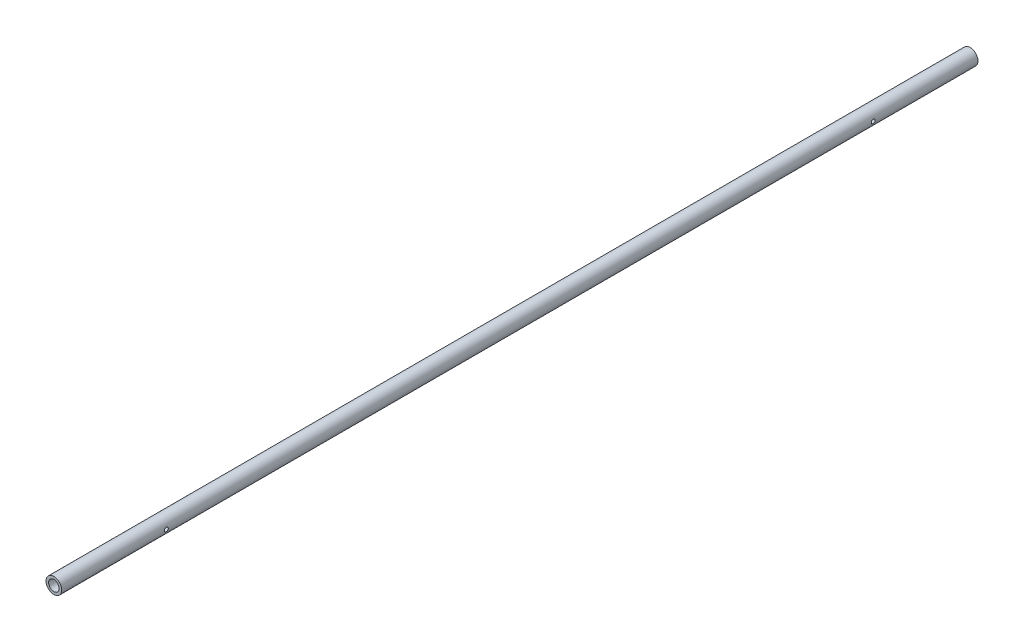
SolidWorks part; units mm, degrees
ref_plane "Front Plane" through (0, 0, 0) normal (0, 0, 1) x (1, 0, 0)
ref_plane "Top Plane" through (0, 0, 0) normal (0, 1, 0) x (1, 0, 0)
ref_plane "Right Plane" through (0, 0, 0) normal (1, 0, 0) x (0, 0, -1)
sketch "Sketch1" plane through (0, 0, 0) normal (0, 0, 1) x (1, 0, 0)
  circle A0 centre (0, 0) radius 2
  circle A1 centre (0, 0) radius 3
  dimension "D1" = 6
  dimension "D2" = 4
extrude "Boss-Extrude1" add sketch "Sketch1" along normal blind 350
sketch "Sketch2" plane through (0, 0, 0) normal (0, 0, -1) x (-1, 0, 0)
  line L0 (0, -3) -> (0, 3) construction
  circle A0 centre (0, 0) radius 3 construction
ref_plane "Plane1" through (0, 0, 0) normal (-1, 0, 0) x (0, 1, 0)
sketch "Sketch3" plane through (0, 0, 0) normal (-1, 0, 0) x (0, 1, 0)
  line L0 (0, 0) -> (0, -350) construction
  line L1 (-2, -350) -> (2, -350) construction
  circle A0 centre (0, -40) radius 0.75
  circle A1 centre (0, -310) radius 0.75
  dimension "D1" = 1.5
  dimension "D3" = 1.5
  dimension "D2" = 40
  dimension "D4" = 40
extrude "Cut-Extrude1" cut sketch "Sketch3" against normal through all and the other way through all
